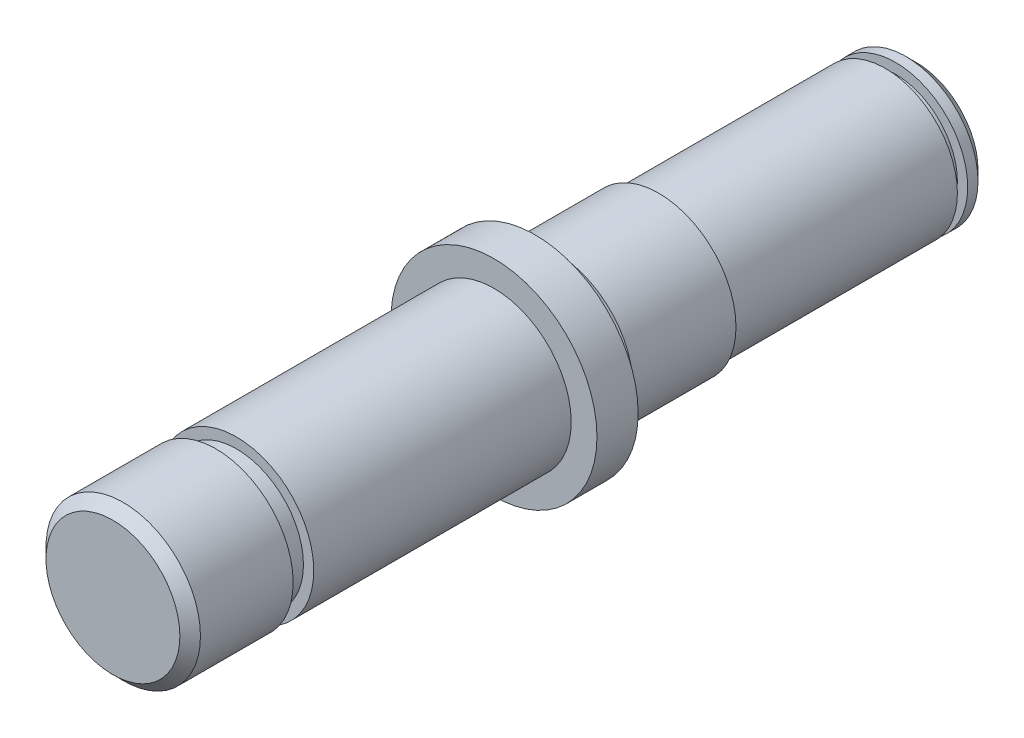
SolidWorks part; units mm, degrees
ref_plane "Front Plane" through (0, 0, 0) normal (0, 0, 1) x (1, 0, 0)
ref_plane "Top Plane" through (0, 0, 0) normal (0, 1, 0) x (1, 0, 0)
ref_plane "Right Plane" through (0, 0, 0) normal (1, 0, 0) x (0, 0, -1)
other "Configuration Table"
sketch "Sketch2" plane through (0, 0, 0) normal (0, 0, 1) x (1, 0, 0)
  circle A0 centre (0, 0) radius 7
  dimension "D1" = 14
extrude "Boss-Extrude1" add sketch "Sketch2" along normal blind 2
sketch "Sketch3" plane through (0, 0, 2) normal (0, 0, 1) x (1, 0, 0)
  circle A0 centre (0, 0) radius 6
  dimension "D1" = 12
extrude "Boss-Extrude2" add sketch "Sketch3" along normal blind 1
sketch "Sketch4" plane through (0, 0, 3) normal (0, 0, 1) x (1, 0, 0)
  circle A1 centre (0, 0) radius 7
  dimension "D1" = 14
extrude "Boss-Extrude3" add sketch "Sketch4" along normal blind 22
sketch "Sketch5" plane through (0, 0, 25) normal (0, 0, 1) x (1, 0, 0)
  circle A0 centre (0, 0) radius 7.5
  dimension "D1" = 15
extrude "Boss-Extrude4" add sketch "Sketch5" along normal blind 10
sketch "Sketch6" plane through (0, 0, 35) normal (0, 0, 1) x (1, 0, 0)
  circle A0 centre (0, 0) radius 6.5
  dimension "D1" = 13
extrude "Boss-Extrude5" add sketch "Sketch6" along normal blind 2
sketch "Sketch7" plane through (0, 0, 37) normal (0, 0, 1) x (1, 0, 0)
  circle A0 centre (0, 0) radius 10
  dimension "D1" = 20
extrude "Boss-Extrude6" add sketch "Sketch7" along normal blind 4
sketch "Sketch8" plane through (0, 0, 41) normal (0, 0, 1) x (1, 0, 0)
  circle A0 centre (0, 0) radius 7.5
  dimension "D1" = 15
extrude "Boss-Extrude7" add sketch "Sketch8" along normal blind 25
sketch "Sketch9" plane through (0, 0, 66) normal (0, 0, 1) x (1, 0, 0)
  circle A0 centre (0, 0) radius 6.5
  dimension "D1" = 13
extrude "Boss-Extrude8" add sketch "Sketch9" along normal blind 2
sketch "Sketch10" plane through (0, 0, 68) normal (0, 0, 1) x (1, 0, 0)
  circle A0 centre (0, 0) radius 7.5
  dimension "D1" = 15
extrude "Boss-Extrude9" add sketch "Sketch10" along normal blind 10
chamfer "Chamfer1" distance 1 angle 45 2 edges at (7, 0, 0) (7.5, 0, 78)
sketch "Sketch11" plane through (0, 0, 0) normal (0, 1, 0) x (1, 0, 0)
  line L0 (0, 0) -> (0, -28.4471)
  line L1 (0, -6.5) -> (0, -19.5) construction
  line L2 (2.5, -6.5) -> (2.5, -19.5)
  line L3 (-2.5, -6.5) -> (-2.5, -19.5)
  line L4 (6, 0) -> (-6, 0) construction
  arc A0 (2.5, -6.5) -> (-2.5, -6.5) centre (0, -6.5) ccw
  arc A1 (-2.5, -19.5) -> (2.5, -19.5) centre (0, -19.5) ccw
  point P5 (0, -13)
  dimension "D1" = 5
  dimension "D2" = 6.5
  dimension "D3" = 13
extrude "Cut-Extrude1" cut sketch "Sketch11" against normal blind 10 from offset 4 contours L0 A1 L2 A0 | L3 A1 L0 A0 offset against normal yes
sketch "Sketch12" plane through (0, 0, 0) normal (0, 1, 0) x (1, 0, 0)
  line L0 (0, 0) -> (0, -82.9296) construction
  line L1 (0, -45.5) -> (0, -58.5) construction
  line L2 (2.5, -45.5) -> (2.5, -58.5)
  line L3 (-2.5, -45.5) -> (-2.5, -58.5)
  line L4 (-6.5, -78) -> (6.5, -78) construction
  arc A0 (2.5, -45.5) -> (-2.5, -45.5) centre (0, -45.5) ccw
  arc A1 (-2.5, -58.5) -> (2.5, -58.5) centre (0, -58.5) ccw
  point P5 (0, -52)
  dimension "D1" = 13
  dimension "D2" = 19.5
  dimension "D3" = 5
extrude "Cut-Extrude2" cut sketch "Sketch12" against normal blind 10 from offset 4.5
